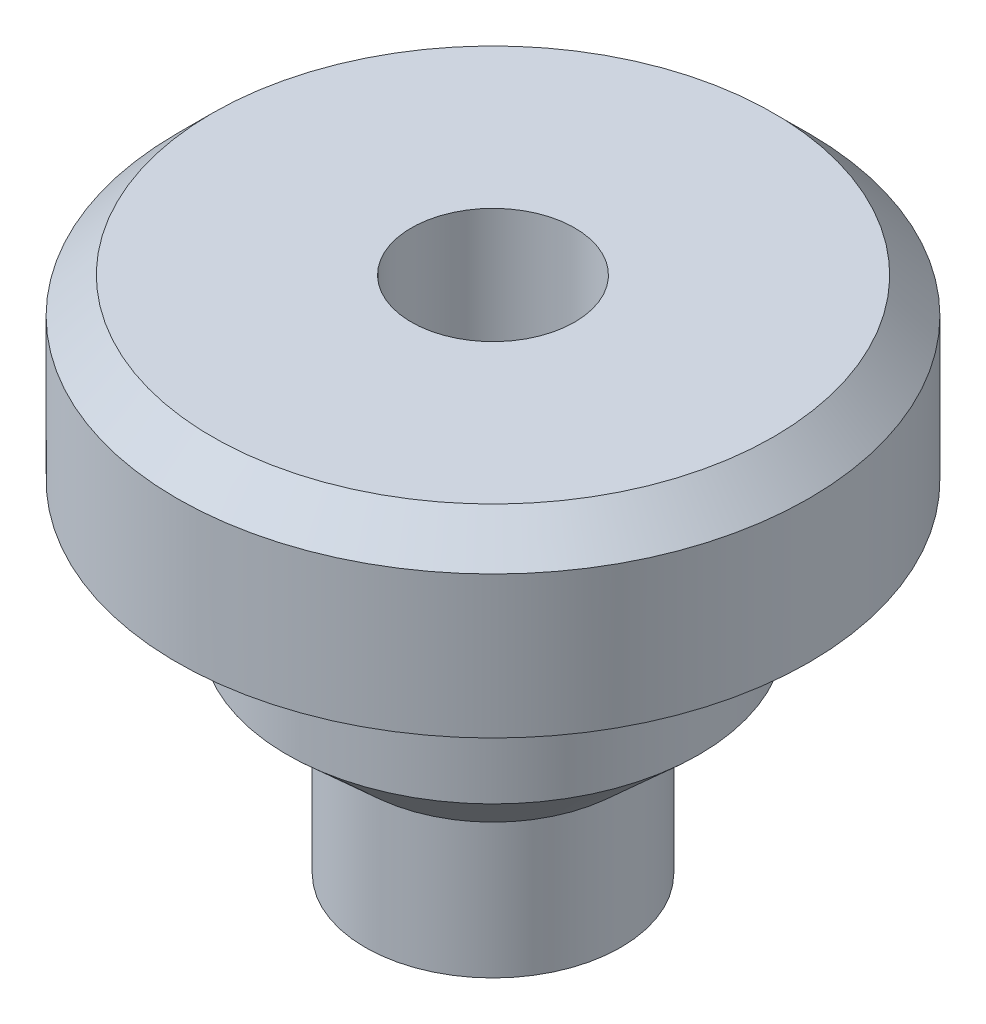
from build123d import *

# Parameters (mm, degrees)
CHAMFER1_SIZE = 5


with BuildPart() as part:
    # Sketch1 → Revolve1 (revolve)
    with BuildSketch(Plane.XY):
        Polygon((11.5, 0), (11.5, 73), (44.5, 73), (44.5, 48), (29, 48), (29, 29), (18, 19), (18, 0), align=None)
    revolve(axis=Axis((0, -693.799212598, 0), (0, 1, 0)))

    # Chamfer1
    chamfer1_edges = [part.edges().sort_by_distance(p)[0] for p in [
        (-44.5, 73, 0),
    ]]
    chamfer(chamfer1_edges, length=CHAMFER1_SIZE)


solid = part.part
